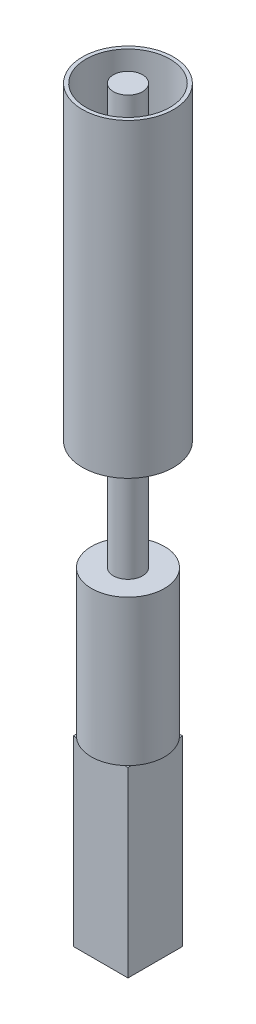
SolidWorks part; units mm, degrees
material "Q235"
ref_plane "Front" through (0, 0, 0) normal (0, 0, 1) x (1, 0, 0)
ref_plane "Top" through (0, 0, 0) normal (0, 1, 0) x (1, 0, 0)
ref_plane "Right" through (0, 0, 0) normal (1, 0, 0) x (0, 0, -1)
sketch "Sketch1" plane through (0, 0, 0) normal (0, 1, 0) x (1, 0, 0)
  circle A0 centre (0, 0) radius 8
  dimension "D1" = 16
extrude "Boss-Extrude1" add sketch "Sketch1" along normal blind 230
sketch "Sketch2" plane through (0, 0, 0) normal (0, 0, 1) x (1, 0, 0)
  line L1 (8, 210) -> (6, 210)
  line L2 (8, 210) -> (8, 230)
  line L3 (8, 230) -> (6, 230)
  line L4 (6, 210) -> (6, 230)
  line L5 (8, 230) -> (-8, 230) construction
  line L6 (8, 0) -> (8, 230) construction
  line L7 (5, 123) -> (11, 123)
  line L8 (5, 123) -> (5, 107)
  line L9 (5, 107) -> (11, 107)
  line L10 (11, 123) -> (11, 107)
  line L11 (5, 123) -> (11, 107) construction
  line L12 (5, 107) -> (11, 123) construction
  point P4 (8, 115)
  dimension "D1" = 20
  dimension "D2" = 2
  dimension "D3" = 1
  dimension "D4" = 16
sketch "Sketch3" plane through (0, 230, 0) normal (0, 1, 0) x (1, 0, 0)
  circle A0 centre (0, 0) radius 25
  circle A1 centre (0, 0) radius 23
  dimension "D1" = 50
  dimension "D2" = 2
extrude "Boss-Extrude2" add sketch "Sketch3" against normal blind 170 separate body
sketch "Sketch4" plane through (0, 0, 0) normal (0, -1, 0) x (1, 0, 0)
  line L1 (-15, 15) -> (15, 15)
  line L2 (-15, 15) -> (-15, -15)
  line L3 (-15, -15) -> (15, -15)
  line L4 (15, 15) -> (15, -15)
  line L5 (-15, 15) -> (15, -15) construction
  line L6 (-15, -15) -> (15, 15) construction
  point P0 (0, 0)
  dimension "D1" = 30
  dimension "D2" = 30
extrude "Boss-Extrude3" add sketch "Sketch4" along normal blind 100 from offset 80
sketch "Sketch5" plane through (0, 0, 0) normal (0, -1, 0) x (1, 0, 0)
  circle A0 centre (0, 0) radius 20
  dimension "D1" = 40
extrude "Boss-Extrude4" add sketch "Sketch5" along normal blind 80
